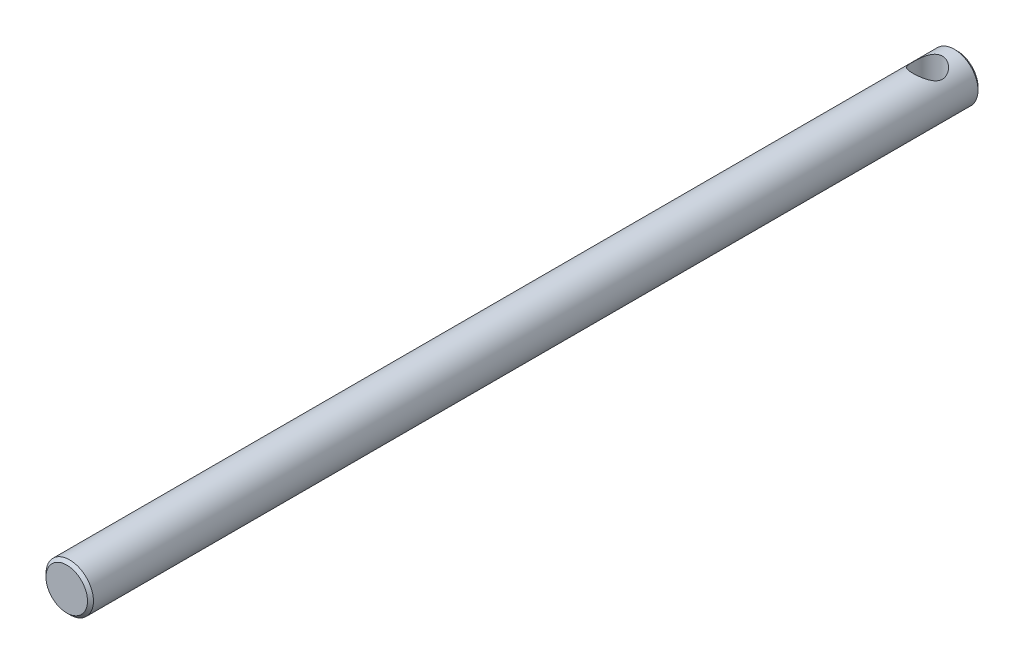
from build123d import *

# Parameters (mm, degrees)
SKETCH1_R           = 4
BOSS_EXTRUDE1_DEPTH = 75
SKETCH2_R           = 2.5
CUT_EXTRUDE1_DEPTH  = 75
CHAMFER1_SIZE       = 0.5


with BuildPart() as part:
    # Sketch1 → Boss-Extrude1 (new, symmetric)
    with BuildSketch(Plane.XY):
        Circle(SKETCH1_R)
    extrude(amount=BOSS_EXTRUDE1_DEPTH, both=True)

    # Sketch2 → Cut-Extrude1 (cut, symmetric)
    with BuildSketch(Plane(origin=(0, 0, 0), x_dir=(1, 0, 0), z_dir=(0, 1, 0))):
        with Locations(Location((0, 70, 0), (0, 0, 270))):
            Circle(SKETCH2_R)
    extrude(amount=CUT_EXTRUDE1_DEPTH, both=True, mode=Mode.SUBTRACT)

    # Chamfer1
    chamfer1_edges = [part.edges().sort_by_distance(p)[0] for p in [
        (-4, 0, -75),
        (-4, 0, 75),
    ]]
    chamfer(chamfer1_edges, length=CHAMFER1_SIZE)


solid = part.part
